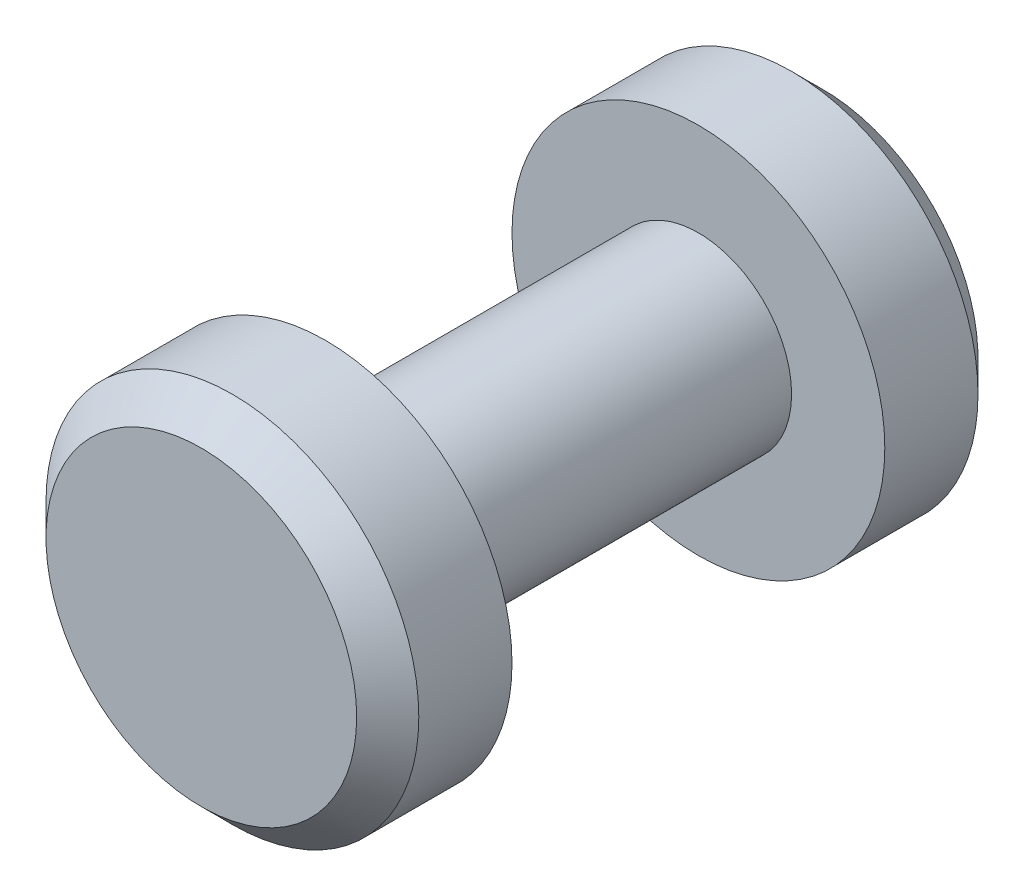
SolidWorks part; units mm, degrees
ref_plane "前视基准面" through (0, 0, 0) normal (0, 0, 1) x (1, 0, 0)
ref_plane "上视基准面" through (0, 0, 0) normal (0, 1, 0) x (1, 0, 0)
ref_plane "右视基准面" through (0, 0, 0) normal (1, 0, 0) x (0, 0, -1)
sketch "草图1" plane through (0, 0, 0) normal (0, 0, 1) x (1, 0, 0)
  circle A0 centre (0, 0) radius 3
extrude "凸台-拉伸1" add sketch "草图1" along normal blind 12
sketch "草图2" plane through (0, 0, 12) normal (0, 0, 1) x (1, 0, 0)
  circle A0 centre (0, 0) radius 6
extrude "凸台-拉伸2" add sketch "草图2" along normal blind 4
chamfer "倒角1" distance 1 angle 45 1 edges at (6, 0, 16)
sketch "草图3" plane through (0, 0, 0) normal (0, 0, -1) x (-1, 0, 0)
  circle A0 centre (0, 0) radius 6
extrude "凸台-拉伸3" add sketch "草图3" along normal blind 4
chamfer "倒角2" distance 1 angle 45 1 edges at (-6, 0, -4)
